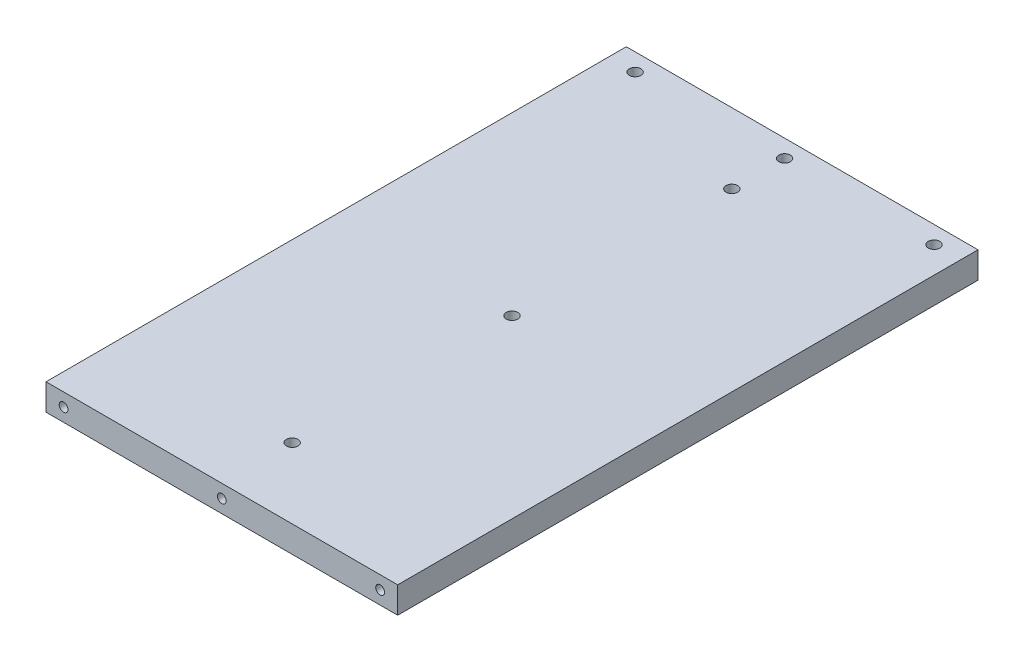
from build123d import *

# Parameters (mm, degrees)
SKETCH_1_W                   = 200
SKETCH_1_H                   = 330
EXTRUDE_1_DEPTH              = 7.5
HOLE_WIZARD_M6_1_D           = 6.6
HOLE_WIZARD_M6_1_CBORE_D     = 11
HOLE_WIZARD_M6_1_CBORE_DEPTH = 8
HOLE_WIZARD_M6_2_D           = 6.6
HOLE_WIZARD_M6_2_CBORE_D     = 11
HOLE_WIZARD_M6_2_CBORE_DEPTH = 8
HOLE_WIZARD_M6_1_2_D         = 5
HOLE_WIZARD_M6_1_2_DEPTH     = 17
HOLE_WIZARD_M6_1_2_TIP       = 1.502151548


with BuildPart() as part:
    # 草图1 → 凸台-拉伸1 (new, symmetric)
    with BuildSketch(Plane(origin=(0, 0, 0), x_dir=(1, 0, 0), z_dir=(0, 1, 0))):
        Rectangle(SKETCH_1_W, SKETCH_1_H)
    extrude(amount=EXTRUDE_1_DEPTH, both=True)

    # Hole Wizard M6 _1 (through all)
    with Locations(Plane(origin=(0, -7.5, 0), x_dir=(-1, 0, 0), z_dir=(0, -1, 0))):
        with Locations((0, 0), (0, -125), (0, 125)):
            CounterBoreHole(HOLE_WIZARD_M6_1_D / 2, HOLE_WIZARD_M6_1_CBORE_D / 2, HOLE_WIZARD_M6_1_CBORE_DEPTH)

    # M6 六角凹头螺钉的柱形沉头孔2 (through all)
    with Locations(Plane(origin=(0, -7.5, 0), x_dir=(-1, 0, 0), z_dir=(0, -1, 0))):
        with Locations((85, 155), (0, 155), (-85, 155)):
            CounterBoreHole(HOLE_WIZARD_M6_2_D / 2, HOLE_WIZARD_M6_2_CBORE_D / 2, HOLE_WIZARD_M6_2_CBORE_DEPTH)

    # Hole Wizard M6 _1 2
    with Locations(Plane.XY.offset(165)):
        with Locations((0, 0), (-90, 0), (90, 0)):
            Hole(HOLE_WIZARD_M6_1_2_D / 2, depth=HOLE_WIZARD_M6_1_2_DEPTH)
            with Locations((0, 0, -(HOLE_WIZARD_M6_1_2_DEPTH + HOLE_WIZARD_M6_1_2_TIP / 2))):  # 118° drill point
                Cone(0, HOLE_WIZARD_M6_1_2_D / 2, HOLE_WIZARD_M6_1_2_TIP, mode=Mode.SUBTRACT)


solid = part.part
